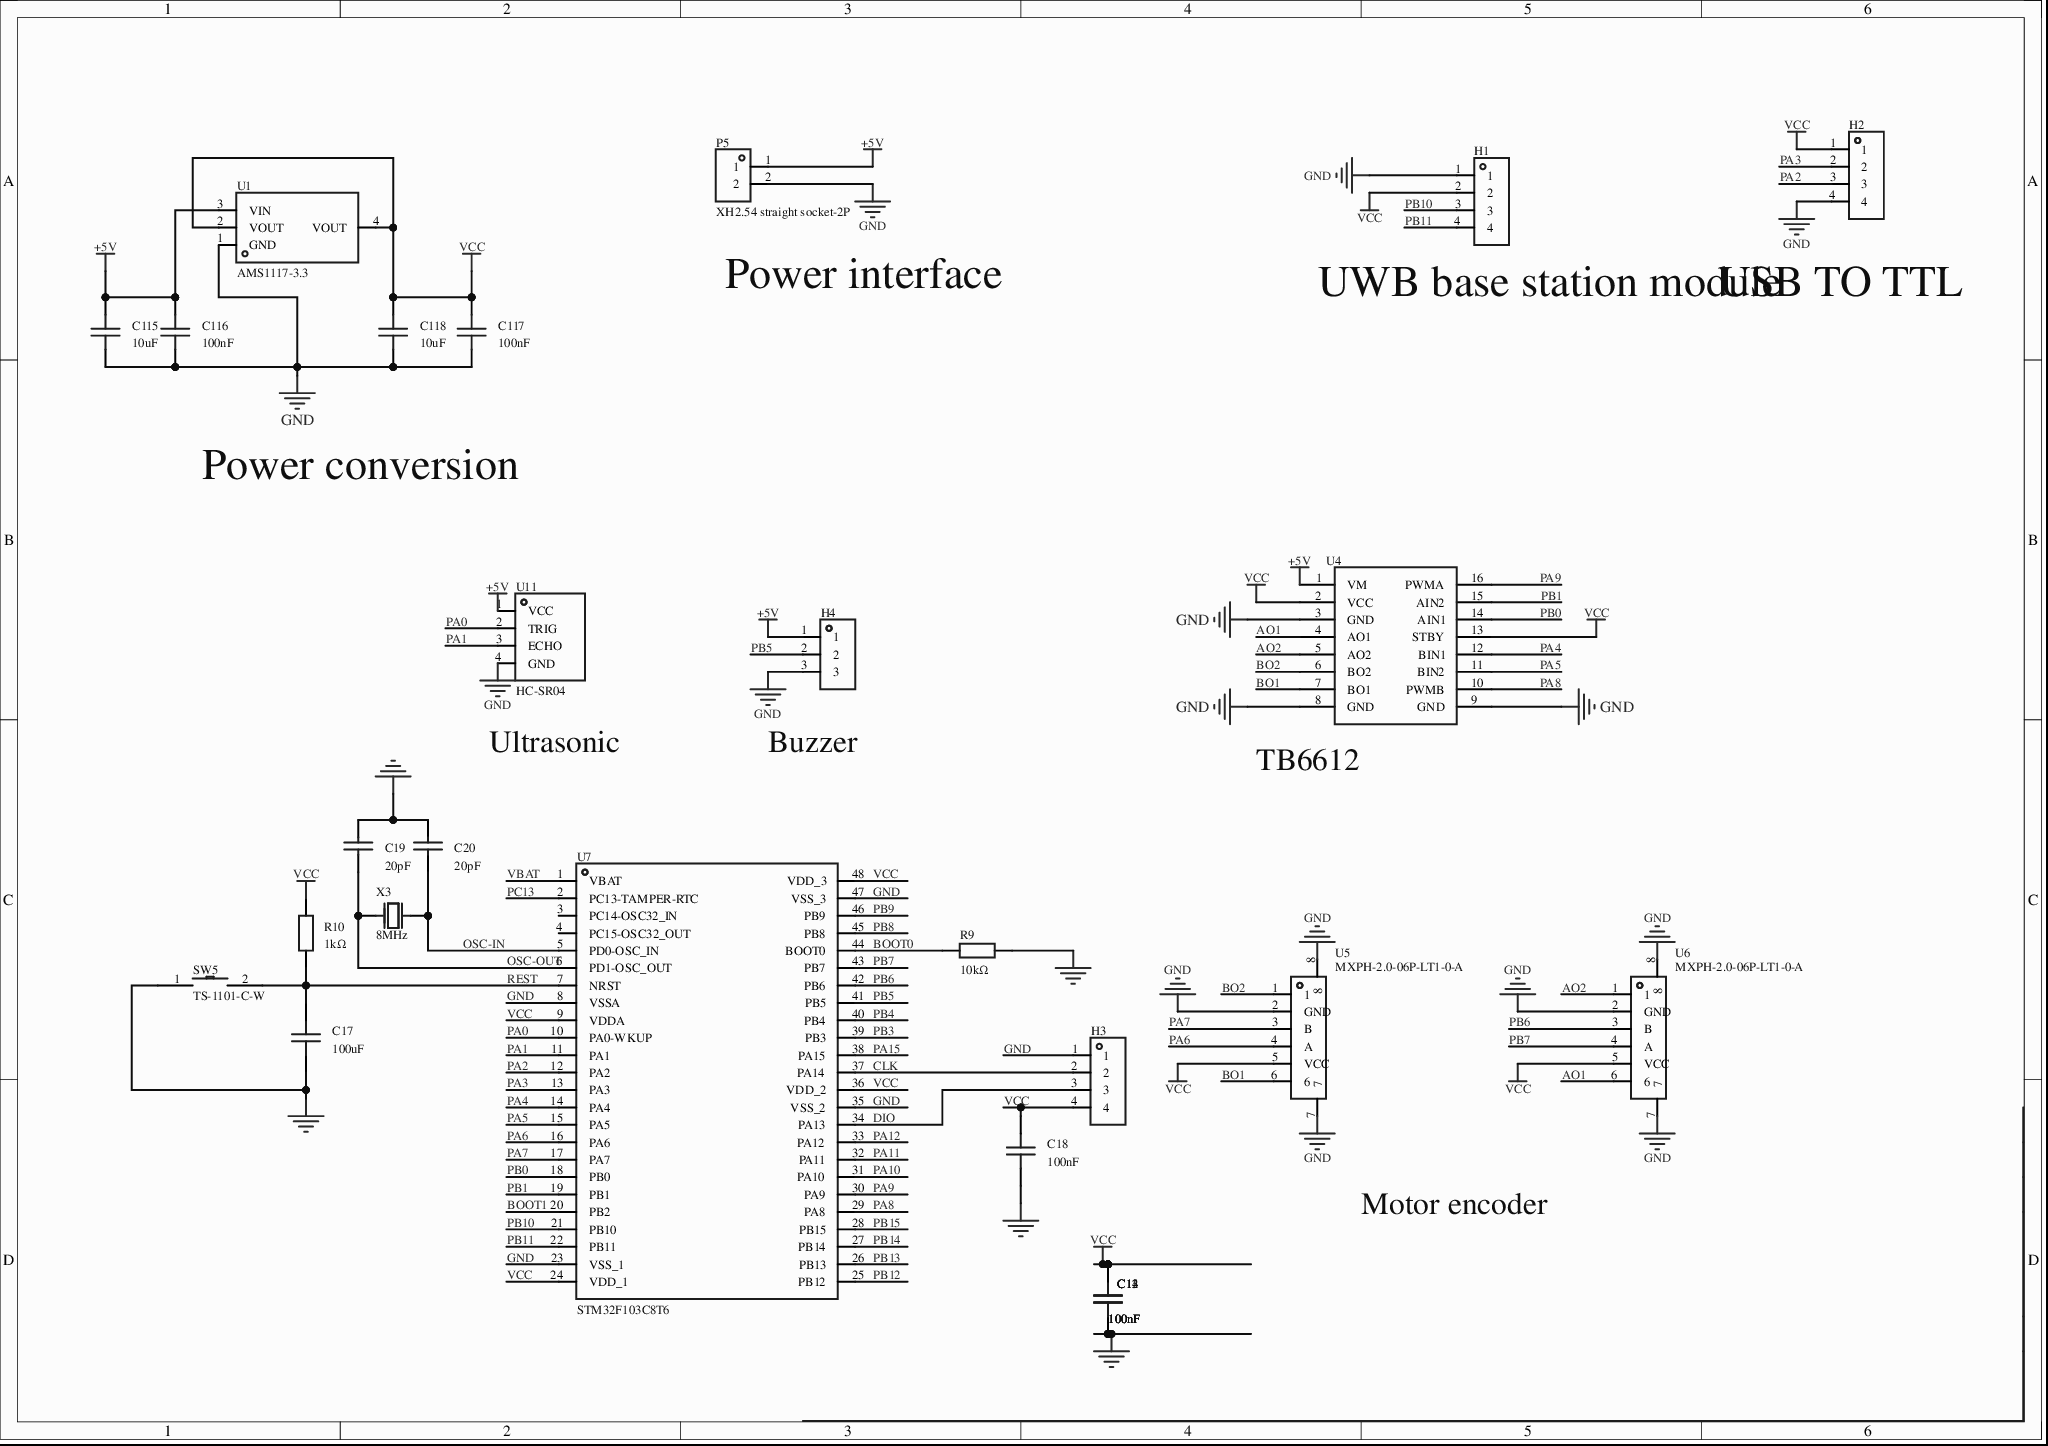
[diagram p0: MISC61262-3.schdoc]
# Altium project MISC61262-2.PrjPcb
1 sheet, 27 parts. Net scope: global (net labels, ports and power ports of the same name join across sheets).
Board file: MISC61262.pcbdoc

## Sheet MISC61262-3.schdoc
size 297 x 209 mm; Version: V1.0; @Project Name: MISC61262; @Page Count: 1; @Update Date: 2026-05-10; @Create Date: 2026-05-10; @Schematic Name: MISC61262; @Page No: 1; @Create Time: 23:22:16; @Update Time: 17:32:40; @Board Name: MISC61262

### Parts
C11  100nF  [C0603]
C12  100nF  [C0603]
C13  100nF  [C0603]
C14  100nF  [C0603]
C17  100uF  [C1206]
C18  100nF  [C0603]
C19  20pF  [C0603]
C20  20pF  [C0603]
C115  10uF  [C0603]
C116  100nF  [C0603]
C117  100nF  [C0603]
C118  10uF  [C0603]
H1  (no value)  [HDR-TH_4P-P2.54-V-M]
H2  (no value)  [HDR-TH_4P-P2.54-V-F]
H3  (no value)  [HDR-TH_4P-P2.54-V-M]
H4  (no value)  [HDR-TH_3P-P2.54-V-F]
P5  XH2.54 straight socket-2P  [CONN-TH_XH2.54-2P]
R9  10kΩ  [R0603]
R10  1kΩ  [R0603]
SW5  TS-1101-C-W  [SW-SMD_L6.0-W3.3-LS8.0]
U1  AMS1117-3.3  [SOT-223-3_L6.5-W3.4-P2.30-LS7.0-BR]
U4  (no value)  [tb6612]
U5  MXPH-2.0-06P-LT1-0-A  [CONN-SMD_6P-P2.00_MXPH-2.0-6P-LT1-0-A]
U6  MXPH-2.0-06P-LT1-0-A  [CONN-SMD_6P-P2.00_MXPH-2.0-6P-LT1-0-A]
U7  STM32F103C8T6  [LQFP-48_L7.0-W7.0-P0.50-LS9.0-BL]
U11  HC-SR04  [TH_HC-SR04V]
X3  8MHz  [OSC-TH_L10.0-W4.5-P5.00]

### Nets
+5V: C115.2 C116.2 H4.1 P5.1 U1.3(VIN) U4.1(VM) U11.1(VCC)
GND: C11.1 C12.1 C13.1 C14.1 C17.1 C18.1 C19.1 C20.1 C115.1 C116.1 C117.1 C118.1 H1.1 H2.4 H3.1 H4.3 P5.2 R9.1 SW5.1 U1.1(GND) U4.3(GND) U4.8(GND) U4.9(GND) U5.2(GND) U5.7 U5.8 U6.2(GND) U6.7 U6.8 U7.8(VSSA) U7.23(VSS_1) U7.35(VSS_2) U7.47(VSS_3) U11.4(GND)
VCC: C11.2 C12.2 C13.2 C14.2 C18.2 C117.2 C118.2 H1.2 H2.1 H3.4 R10.2 U1.2(VOUT) U1.4(VOUT) U4.2(VCC) U4.13(STBY) U5.5(VCC) U6.5(VCC) U7.9(VDDA) U7.24(VDD_1) U7.36(VDD_2) U7.48(VDD_3)
AO1: U4.4(AO1) U6.6
AO2: U4.5(AO2) U6.1
BO1: U4.7(BO1) U5.6
BO2: U4.6(BO2) U5.1
BOOT0: R9.2 U7.44(BOOT0)
BOOT1: U7.20(PB2)
CLK: H3.2 U7.37(PA14)
DIO: H3.3 U7.34(PA13)
OSC-IN: C20.2 U7.5(PD0-OSC_IN) X3.1(OSC1)
OSC-OUT: C19.2 U7.6(PD1-OSC_OUT) X3.2(OSC2)
PA0: U7.10(PA0-WKUP) U11.2(TRIG)
PA1: U7.11(PA1) U11.3(ECHO)
PA2: H2.3 U7.12(PA2)
PA3: H2.2 U7.13(PA3)
PA4: U4.12(BIN1) U7.14(PA4)
PA5: U4.11(BIN2) U7.15(PA5)
PA6: U5.4(A) U7.16(PA6)
PA7: U5.3(B) U7.17(PA7)
PA8: U4.10(PWMB) U7.29(PA8)
PA9: U4.16(PWMA) U7.30(PA9)
PA10: U7.31(PA10)
PA11: U7.32(PA11)
PA12: U7.33(PA12)
PA15: U7.38(PA15)
PB0: U4.14(AIN1) U7.18(PB0)
PB1: U4.15(AIN2) U7.19(PB1)
PB3: U7.39(PB3)
PB4: U7.40(PB4)
PB5: H4.2 U7.41(PB5)
PB6: U6.3(B) U7.42(PB6)
PB7: U6.4(A) U7.43(PB7)
PB8: U7.45(PB8)
PB9: U7.46(PB9)
PB10: H1.3 U7.21(PB10)
PB11: H1.4 U7.22(PB11)
PB12: U7.25(PB12)
PB13: U7.26(PB13)
PB14: U7.27(PB14)
PB15: U7.28(PB15)
PC13: U7.2(PC13-TAMPER-RTC)
REST: C17.2 R10.1 SW5.2 U7.7(NRST)
VBAT: U7.1(VBAT)

Not connected (* = marked no-connect by the designer): U7 3(PC14-OSC32_IN) 4(PC15-OSC32_OUT)

### Notes on the sheet
- (near P5) Power interface
- (near H1) UWB base station module
- (near H2) USB TO TTL
- Power conversion
- 串口：
  UWB基站  		PB11，PB10 	(UART3）
  USB TO TTL     PA2,PA3        (UART2)
  GPIO:
  超声波  PA1
  蜂鸣器  PB5
  TB6612  BINT1  PA4
  TB6612  BINT2  PA5
  TB6612  AINT2  PB1
  TB6612  AINT1  PB0
  TIM:
  超声波 PA0 （TIM2_CH1）
  TB6612  PWMA  PA9 (TIM1_CH2)
  TB6612  PWMB  PA8 (TIM1_CH1)
  右编码器  编码器信号线B相  PA7 (TIM3_CH2)
  右编码器  编码器信号线A相  PA6 (TIM3_CH1)
  左编码器  编码器信号线B相  PB6 (TIM4_CH1)
  左编码器  编码器信号线A相  PB7 (TIM4_CH2)
  编码器的M和P：
  右编码器  电机电源线M  接到TB6612的B01
  右编码器  电机电源线P   接到TB6612的B02
  左编码器  电机电源线M  接到TB6612的A02
  左编码器  电机电源线P   接到TB6612的A01
  供电：
  TB6612模块 VM接5V
  STM32F103C8T6 5V接5V
  超声波    VCC接3.3V，    3.3V由MCU提供
  UWB基站 VCC接3.3V      3.3V由MCU提供
  蜂鸣器    VCC接3.3V      3.3V由MCU提供
  串口模块图片如下：
- (near U11) Ultrasonic
- (near H4) Buzzer
- (near U4) TB6612
- Motor encoder

### Library data of the parts
C11-C14 C18 = CGA0603X7R104K500JT: Capacitance: 100nF; tolerance: ±10%; rated voltage: 50V; dielectric (temperature coefficient): X7R;; Manufacturer: HRE(芯声); 3D Model: ac125912035d415993ca9572d50418b1; 3D Model Transform: 62.992,31.496,0,0,0,0,0,0,0; AddInBom: yes; ModelName: C0603_L1.6-W0.8-H0.8; Symbol: CGA0603X7R104K500JT; Device: CGA0603X7R104K500JT; LCSC Part Name: 100nF ±10% 50V; Supplier Part: C6119867; Manufacturer Part: CGA0603X7R104K500JT; Supplier Footprint: 0603; JLCPCB Part Class: Extended library; Supplier: LCSC; Value: 100nF; Tolerance: ±10%; Voltage Rated: 50V; Temperature Coefficient: X7R; ConvertToPcb: yes; FootprintName: C0603
C17 = HGC1206R5107M100NSPJ: Capacitance: 100uF; tolerance: ±20%; rated voltage: 10V; dielectric (temperature coefficient): X5R;; Manufacturer: Chinocera(华瓷); 3D Model: e4be705b945545a48e666415e3682bd8; 3D Model Transform: 125.984,62.992,0,0,0,0,0,0,0; AddInBom: yes; ModelName: C1206_L3.2-W1.6-H1.3; Symbol: HGC1206R5107M100NSPJ; Device: HGC1206R5107M100NSPJ; LCSC Part Name: 100uF ±20% 10V; Supplier Part: C7432784; Manufacturer Part: HGC1206R5107M100NSPJ; Supplier Footprint: 1206; JLCPCB Part Class: Extended library; Datasheet: https://atta.szlcsc.com/upload/public/pdf/source/20240320/FAC3FEC40A78BC5CCCE96C232A94D860.pdf; Supplier: LCSC; Value: 100uF; Tolerance: ±20%; Voltage Rated: 10V; Temperature Coefficient: X5R; ConvertToPcb: yes; FootprintName: C1206
C19 C20 = CL10C200JB8NNNC: Capacitance: 20pF; tolerance: ±5%; rated voltage: 50V; dielectric (temperature coefficient): C0G;; Manufacturer: SAMSUNG(三星); 3D Model: ac125912035d415993ca9572d50418b1; 3D Model Transform: 62.992,31.496,0,0,0,0,0,0,0; AddInBom: yes; ModelName: C0603_L1.6-W0.8-H0.8; Symbol: CL10C200JB8NNNC; Device: CL10C200JB8NNNC; LCSC Part Name: 20pF ±5% 50V; Supplier Part: C1648; Manufacturer Part: CL10C200JB8NNNC; Supplier Footprint: 0603; JLCPCB Part Class: Basic library; Datasheet: https://atta.szlcsc.com/upload/public/pdf/source/20160218/1457707763339.pdf; Supplier: LCSC; Value: 20pF; Tolerance: ±5%; Voltage Rated: 50V; Temperature Coefficient: C0G; ConvertToPcb: yes; FootprintName: C0603
C115 C118 = CL10A106KP8NNNC: Capacitance: 10uF; tolerance: ±10%; rated voltage: 10V; dielectric (temperature coefficient): X5R;; Manufacturer: SAMSUNG(三星); 3D Model: ac125912035d415993ca9572d50418b1; 3D Model Transform: 62.992,31.496,0,0,0,0,0,0,0; AddInBom: yes; ModelName: C0603_L1.6-W0.8-H0.8; Symbol: CL10A106KP8NNNC; Device: CL10A106KP8NNNC; LCSC Part Name: 10uF ±10% 10V; Supplier Part: C19702; Manufacturer Part: CL10A106KP8NNNC; Supplier Footprint: 0603; JLCPCB Part Class: Basic library; Datasheet: https://atta.szlcsc.com/upload/public/pdf/source/20160103/1457707703378.pdf; Supplier: LCSC; Value: 10uF; Tolerance: ±10%; Voltage Rated: 10V; Temperature Coefficient: X5R; ConvertToPcb: yes; FootprintName: C0603
C116 C117 = CC0603KRX7R9BB104: Capacitance: 100nF; tolerance: ±10%; rated voltage: 50V; dielectric (temperature coefficient): X7R;; Manufacturer: YAGEO(国巨); 3D Model: ac125912035d415993ca9572d50418b1; 3D Model Transform: 62.992,31.496,0,0,0,0,0,0,0; AddInBom: yes; ModelName: C0603_L1.6-W0.8-H0.8; Symbol: CC0603KRX7R9BB104; Device: CC0603KRX7R9BB104; LCSC Part Name: 100nF ±10% 50V; Supplier Part: C14663; Manufacturer Part: CC0603KRX7R9BB104; Supplier Footprint: 0603; JLCPCB Part Class: Basic library; Datasheet: https://atta.szlcsc.com/upload/public/pdf/source/20180910/C282072_33301C7F631E79921B82A8DAC6BCC5B3.pdf; Supplier: LCSC; Value: 100nF; Tolerance: ±10%; Voltage Rated: 50V; Temperature Coefficient: X7R; ConvertToPcb: yes; FootprintName: C0603
H1 = HDR-M_2.54_1x4P: Symbol: PZ254V-11-04P; ConvertToPcb: yes; ModelId: 112f4d05e8d64e99ab9a333894bea4f90819f05c4eef4c71ace90d822a990e87; ModelName: HDR-TH_4P-P2.54-M-LI-1X4P; ModelTransform: 399.999,104.7242,0,0,0,0,0,0,-118.11; Device: HDR-M_2.54_1x4P; AddInBom: yes; SupplierPart: C492403; Supplier Footprint: 插件; FootprintName: HDR-TH_4P-P2.54-V-M
H2 = HDR-F_2.54_1x4P: Symbol: 2.54-1*4P female; ConvertToPcb: yes; ModelId: d187812051054f85879fcaa51a310d8e0819f05c4eef4c71ace90d822a990e87; ModelTransform: 419.6842,98.464,0,0,0,0,0,0,-118.11; Device: HDR-F_2.54_1x4P; AddInBom: yes; SupplierPart: C2718488; Supplier Footprint: 插件; FootprintName: HDR-TH_4P-P2.54-V-F; ModelName: HDR-TH_4P-P2.54-V-F
H3 = HDR-M_2.54_1x4P: Symbol: PZ254V-11-04P; 3D Model: 112f4d05e8d64e99ab9a333894bea4f90819f05c4eef4c71ace90d822a990e87; 3D Model Transform: 399.999,104.7242,0,0,0,0,0,0,-118.11; ConvertToPcb: yes; ModelName: HDR-TH_4P-P2.54-M-LI-1X4P; Device: HDR-M_2.54_1x4P; Supplier Part: C492403; Supplier Footprint: 插件; AddInBom: yes; FootprintName: HDR-TH_4P-P2.54-V-M
H4 = HDR-F_2.54_1x3P: Symbol: PM254V-11-03-H85; ConvertToPcb: yes; ModelId: f3b3cc5aae9641bf9e56fc160cef875b; ModelName: HDR2.54-F-LI-1X3P; ModelTransform: 299.9994,100,0,0,0,0,0,0,-118.11; Device: HDR-F_2.54_1x3P; AddInBom: yes; SupplierPart: C541850; Supplier Footprint: 插件; FootprintName: HDR-TH_3P-P2.54-V-F
P5 = XH2.54直插座-2P: 3D Model: c3cc11bd8b8748c1ae6bc231aac3a1ff0819f05c4eef4c71ace90d822a990e87; 3D Model Transform: 296.889,230.315,0,0,0,0,0,26.653,-137.795; AddInBom: yes; Symbol: XH2.54 straight socket-2P; Device: XH2.54 straight socket-2P; LCSC Part Name: XH2.54直插座-2P; Supplier Part: C9900016957; Manufacturer Part: XH2.54直插座-2P; Supplier Footprint: XH2.54-2; JLCPCB Part Class: Extended Part; Supplier: LCSC; ConvertToPcb: yes; FootprintName: CONN-TH_XH2.54-2P; ModelName: CONN-TH_XH2.54-2P
R9 = 0603WAF1002T5E: Resistor type: thick film resistor; resistance: 10kΩ; tolerance: ±1%; power: 100mW; max working voltage: 75V; temperature coefficient: ±100ppm/℃;; Manufacturer: UNI-ROYAL(厚声); 3D Model: fc143cca1e79419f9cd78b61e9279f08; 3D Model Transform: 31.8897,63.7794,0,90,0,0,0,0,0; AddInBom: yes; Symbol: 0603WAF1002T5E; Device: 0603WAF1002T5E; LCSC Part Name: 厚膜电阻 10kΩ ±1% 100mW; Supplier Part: C25804; Manufacturer Part: 0603WAF1002T5E; Supplier Footprint: 0603; JLCPCB Part Class: Basic library; Datasheet: https://atta.szlcsc.com/upload/public/pdf/source/20200306/C422600_1E6D84923E4A46A82E41ADD87F860B5C.pdf; Supplier: LCSC; Type: Thick film resistor; Value: 10kΩ; Tolerance: ±1%; Power(Watts): 100mW; Overload Voltage (Max): 75V; Temperature Coefficient: ±100ppm/℃; Operating Temperature Range: -55℃~+155℃; ConvertToPcb: yes; FootprintName: R0603; ModelName: R0603
R10 = RC0603FR-071KL: Resistor type: thick film resistor; resistance: 1kΩ; tolerance: ±1%; power: 100mW; max working voltage: 75V; temperature coefficient: ±100ppm/℃;; Manufacturer: YAGEO(国巨); 3D Model: fc143cca1e79419f9cd78b61e9279f08; 3D Model Transform: 31.8897,63.7794,0,90,0,0,0,0,0; AddInBom: yes; Symbol: RC0603FR-071KL; Device: RC0603FR-071KL; LCSC Part Name: 厚膜电阻 1kΩ ±1% 100mW; Supplier Part: C22548; Manufacturer Part: RC0603FR-071KL; Supplier Footprint: 0603; JLCPCB Part Class: Extended library; Datasheet: https://atta.szlcsc.com/upload/public/pdf/source/20180316/70C0E2BDAE7FCC62C531A5A58D202EE1.pdf; Supplier: LCSC; Type: Thick film resistor; Value: 1kΩ; Tolerance: ±1%; Power(Watts): 100mW; Overload Voltage (Max): 75V; Temperature Coefficient: ±100ppm/℃; Operating Temperature Range: -55℃~+155℃; ConvertToPcb: yes; FootprintName: R0603; ModelName: R0603
SW5 = TS-1101-C-W: 电路结构:单刀单掷;按钮形状:矩形按钮;作用力:260gf;安装方式:立贴;开关长度:6mm;开关宽度:3.6mm;开关高度:2.5mm;带支架:不带;触点电流:50mA;额定电压(AC):-;额定电压(DC):12V;额定功率:-;绝缘电阻:-;带灯:无;机械寿命:5万次;; Manufacturer: XKB Connectivity(中国星坤); 3D Model: b2f4ea9f0afc4b0786d53dba66ceb9e4; 3D Model Transform: 314.96,129.921,0,0,0,0,0,0,0; Circuit: SPST; Actuator Style: Rectangular button; Operating Force: 260gf; Switch Length: 6mm; Switch Width: 3.6mm; Switch Height: 2.5mm; Strike Gundam: No; Contact Current: 50mA; Voltage Rating (DC): 12V; Actuator/Cap Color: White with light green; With Lamp: None; Mechanical Life: 5万 cycles; AddInBom: yes; ModelName: SW-SMD_L6.0-W3.3-H5-LS8.0; Symbol: TS-1101-C-W; Device: TS-1101-C-W; LCSC Part Name: 6*3.6*2.5mm 立贴 轻触开关; Supplier Part: C318938; Manufacturer Part: TS-1101-C-W; Supplier Footprint: SMD; JLCPCB Part Class: Extended library; Datasheet: https://atta.szlcsc.com/upload/public/pdf/source/20200227/C318938_C2E53B1EEDE37D980A33616AC086DE53.pdf; Supplier: LCSC; Mounting Style: Surface mount; Voltage Rating (AC): -; Power Rating: -; Insulation Resistance: -; IP Rating: -; Pin Style: -; Operating Temperature: -30℃~+85℃; ConvertToPcb: yes; FootprintName: SW-SMD_L6.0-W3.3-LS8.0
U1 = AMS1117-3.3_C6186: Output type: fixed; working voltage: -; output voltage: 3.3V; output current: 1A; power supply ripple rejection ratio (PSRR): 72dB@(120Hz); output polarity: positive;; Manufacturer: AMS; AddInBom: yes; ModelId: 925194bf9823436183a3e0b978a8d076; ModelName: SOT-223-4P_L6.5-W3.5-H1.6-LS7.0-P2.30; ModelTransform: 279.89794,255.905,0,180,0,0,-3.9385,-0.0005,0; Voltage Dropout: 1.3V@(800mA); Number of Outputs: 1; Symbol: AMS1117-3.3; Device: AMS1117-3.3_C6186; LCSC Part Name: 输出3.3V 1A; SupplierPart: C6186; ManufacturerPart: AMS1117-3.3; Supplier Footprint: SOT-223; Datasheet: https://atta.szlcsc.com/upload/public/pdf/source/20180727/C6186_7A095716F0823C02F1997A905E26C086.pdf; Supplier: LCSC; ConvertToPcb: yes; FootprintName: SOT-223-3_L6.5-W3.4-P2.30-LS7.0-BR; Output Type: Fixed; Voltage - Supply: -; Output Voltage: 3.3V; Output Current: 1A; Power Supply Rejection Ratio (PSRR): 72dB@(120Hz); standby current: -; Noise: -; Features: Overcurrent protection (OCP); thermal shutdown (TSD); Operating Temperature: -; Output Configuration: Positive
U4 = tb6612: AddInBom: yes; Symbol: tb6612; Device: tb6612; JLCPCB Part Class: Extended library; ConvertToPcb: yes; FootprintName: tb6612
U5 = MXPH-2.0-06P-LT1-0-A: 插针结构:1x6P;间距:2mm;安装方式:立贴;参考系列:PH;总PIN数:6P;排数:1;每排PIN数:6;额定电流:2A;触头材质:铜合金;触头镀层:锡;工作温度:-25℃~+85℃;; Manufacturer: MAX(迈旭); Symbol: MXPH-2.0-06P-LT1-0-A_1; AddInBom: yes; ModelId: 7656877d212b4dcda05e79af15a508d50819f05c4eef4c71ace90d822a990e87; ModelTransform: 629.92,281.4955,0,180,0,0,0,26.22,0; Pins Structure: 1x6P; Pitch: 2mm; Reference Series: PH; Number of PINs Per Row: 6; Current Rating: 2A; Voltage Rating: 250V; Plastic Material: LCP; Flame Retardant Rating: UL94V-0; Device: MXPH-2.0-06P-LT1-0-A; LCSC Part Name: 象牙白 1x6P 间距:2mm 立贴 系列:PH; SupplierPart: C7542145; ManufacturerPart: MXPH-2.0-06P-LT1-0-A; Supplier Footprint: SMD,P=2mm; JLCPCB Part Class: Extended Part; Datasheet: https://item.szlcsc.com/datasheet/MXPH-2.0-06P-LT1-0-A/8645846.html; Supplier: LCSC; ConvertToPcb: yes; FootprintName: CONN-SMD_6P-P2.00_MXPH-2.0-6P-LT1-0-A; ModelName: CONN-SMD_6P-P2.00_MXPH-2.0-6P-LT1-0-A; Mounting Type: Surface mount; Number of Pins: 6P; Number of Rows: 1; Contact Material: Copper alloy; Contact Plating: Tin; Operating Temperature: -25℃~+85℃; Color: -
U6 = MXPH-2.0-06P-LT1-0-A: 插针结构:1x6P;间距:2mm;安装方式:立贴;参考系列:PH;总PIN数:6P;排数:1;每排PIN数:6;额定电流:2A;触头材质:铜合金;触头镀层:锡;工作温度:-25℃~+85℃;; Manufacturer: MAX(迈旭); Symbol: MXPH-2.0-06P-LT1-0-A_1; 3D Model: 7656877d212b4dcda05e79af15a508d50819f05c4eef4c71ace90d822a990e87; 3D Model Transform: 629.92,281.4955,0,180,0,0,0,26.22,0; Pins Structure: 1x6P; Pitch: 2mm; Reference Series: PH; Number of PINs Per Row: 6; Current Rating: 2A; Voltage Rating: 250V; Plastic Material: LCP; Flame Retardant Rating: UL94V-0; AddInBom: yes; Device: MXPH-2.0-06P-LT1-0-A; LCSC Part Name: 象牙白 1x6P 间距:2mm 立贴 系列:PH; Supplier Part: C7542145; Manufacturer Part: MXPH-2.0-06P-LT1-0-A; Supplier Footprint: SMD,P=2mm; JLCPCB Part Class: Extended Part; Datasheet: https://item.szlcsc.com/datasheet/MXPH-2.0-06P-LT1-0-A/8645846.html; Supplier: LCSC; Mounting Type: Surface mount; Number of Pins: 6P; Number of Rows: 1; Contact Material: Copper alloy; Contact Plating: Tin; Operating Temperature: -25℃~+85℃; Color: -; ConvertToPcb: yes; FootprintName: CONN-SMD_6P-P2.00_MXPH-2.0-6P-LT1-0-A; ModelName: CONN-SMD_6P-P2.00_MXPH-2.0-6P-LT1-0-A
U7 = STM32F103C8T6: CPU内核:ARM-M3;程序存储容量:64KB;RAM总容量:20KB;GPIO端口数量:37;工作电压范围:2V~3.6V;CPU最大主频:72MHz;程序存储器类型:FLASH;; Manufacturer: ST(意法半导体); 3D Model: 093be70396ff421eb2cdb946d5311efc; 3D Model Transform: 354.331,354.331,0,0,0,0,0,0,0; CPU Core: ARM-M3; Program Storage Size: 64KB; RAM Size: 20KB; GPIO Ports Number: 37; CPU Maximum Speed: 72MHz; Program Memory Type: FLASH; ADC (Bit): 12bit; Universal Serial Bus: Yes; Peripheral/Function: Watchdog; DMA; watchdog; temperature sensor; ModelName: LQFP-48_L7.0-W7.0-H1.4-LS9.0-P0.50; Symbol: STM32F103C8T6; Device: STM32F103C8T6; LCSC Part Name: 主流增强型ARM Cortex-M3 MCU，具有64 KB Flash、72 MHz CPU、电机控制、USB和CAN; Supplier Part: C8734; Manufacturer Part: STM32F103C8T6; Supplier Footprint: LQFP-48(7x7); JLCPCB Part Class: Extended library; Datasheet: https://atta.szlcsc.com/upload/public/pdf/source/20220812/8363ACEC51AD55ECEB84799464F7CB85.pdf; Supplier: LCSC; Operating Voltage Range: 2V~3.6V; Operating Temperature Range: -40℃~+85℃; DAC (Bit): -; PWM (Bit): -; Internal Comparator: -; communication protocol: -; Watchdog: Yes; Real-Time Clock: -; Infrared Data Association: Yes; Low-Voltage Detect: Yes; CCP Capture/Compare: -; Secure Digital Input and Output: -; Direct Memory Access: Yes; Internal Oscillator: Yes; AddInBom: yes; ConvertToPcb: yes; FootprintName: LQFP-48_L7.0-W7.0-P0.50-LS9.0-BL
U11 = HC-SR04: Manufacturer: Universal Microelectronics; AddInBom: yes; Symbol: HC-SR04; Device: HC-SR04; LCSC Part Name: HC-SR04; SupplierPart: C19857336; ManufacturerPart: HC-SR04; Supplier Footprint: -; JLCPCB Part Class: Extended library; Datasheet: https://atta.szlcsc.com/upload/public/pdf/source/20240122/47B8E374E428935B7962A2189EF91AAC.pdf; Supplier: LCSC; ConvertToPcb: yes; FootprintName: TH_HC-SR04V
X3 = X49SD8MSD2SC: Crystal type: through-hole crystal; frequency: 8MHz; frequency deviation at room temperature: ±20ppm; external load capacitance: 20pF; frequency stability (full temperature): ±30ppm;; Manufacturer: YXC(扬兴晶振); 3D Model: a8e34f6c394c4d60ace7720f62d1ccdf; 3D Model Transform: 432.46488,177.165,0,90,0,0,0,0,-137.795; AddInBom: yes; ModelName: HC-49US_L11.0-W4.5-H3.5-P4.88; Symbol: X49SD8MSD2SC; Device: X49SD8MSD2SC; LCSC Part Name: 8MHz ±20ppm 20pF; Supplier Part: C21263; Manufacturer Part: X49SD8MSD2SC; Supplier Footprint: HC-49S; JLCPCB Part Class: Extended library; Datasheet: https://atta.szlcsc.com/upload/public/pdf/source/20240329/977D7F2434F98B2BE33270BB9FF3D86D.pdf; Supplier: LCSC; Crystal Type: Through-hole crystal; Value: 8MHz; Normal temperature Frequency Tolerance: ±20ppm; External load capacitor: 20pF; Frequency Stability(Full temperature range): ±30ppm; Operating Temperature: -20℃~+70℃; ConvertToPcb: yes; FootprintName: OSC-TH_L10.0-W4.5-P5.00